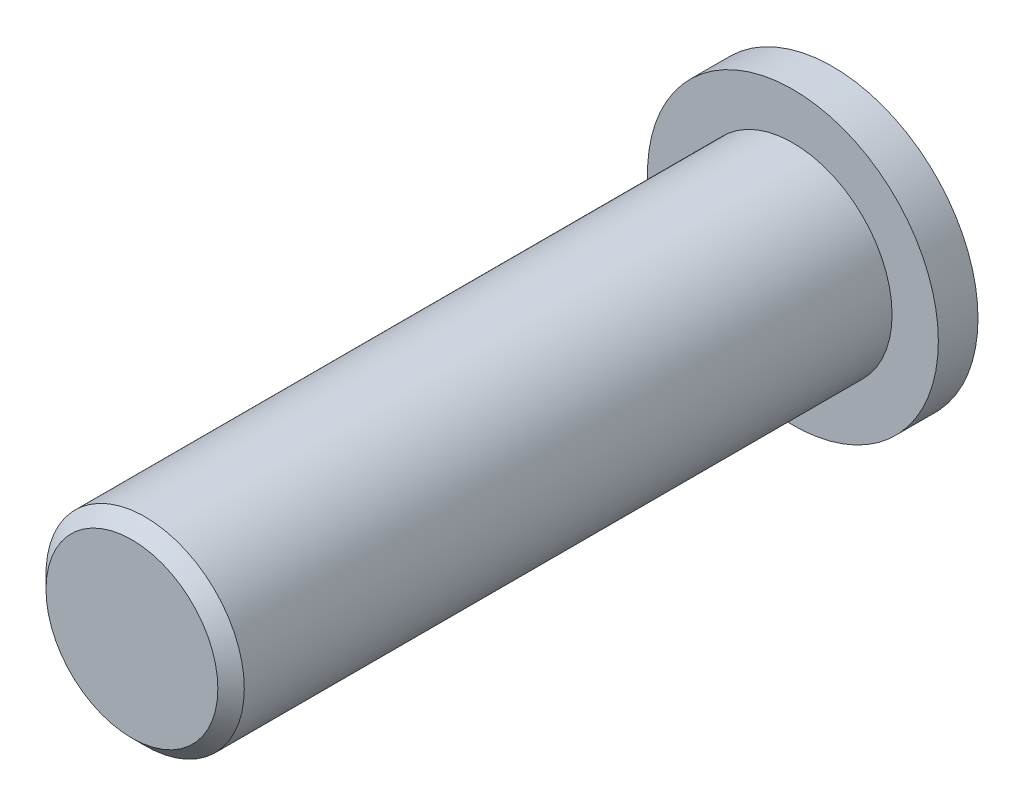
SolidWorks part; units mm, degrees
ref_plane "前视基准面" through (0, 0, 0) normal (0, 0, 1) x (1, 0, 0)
ref_plane "上视基准面" through (0, 0, 0) normal (0, 1, 0) x (1, 0, 0)
ref_plane "右视基准面" through (0, 0, 0) normal (1, 0, 0) x (0, 0, -1)
other "Configuration Table"
sketch "草图1" plane through (0, 0, 0) normal (0, 0, 1) x (1, 0, 0)
  circle A0 centre (0, 0) radius 11
  dimension "D1" = 22
extrude "凸台-拉伸1" add sketch "草图1" along normal blind 3
sketch "草图2" plane through (0, 0, 3) normal (0, 0, 1) x (1, 0, 0)
  circle A0 centre (0, 0) radius 7.5
  dimension "D1" = 15
extrude "凸台-拉伸2" add sketch "草图2" along normal blind 50
chamfer "倒角1" distance 1 angle 45 1 edges at (7.5, 0, 53)
